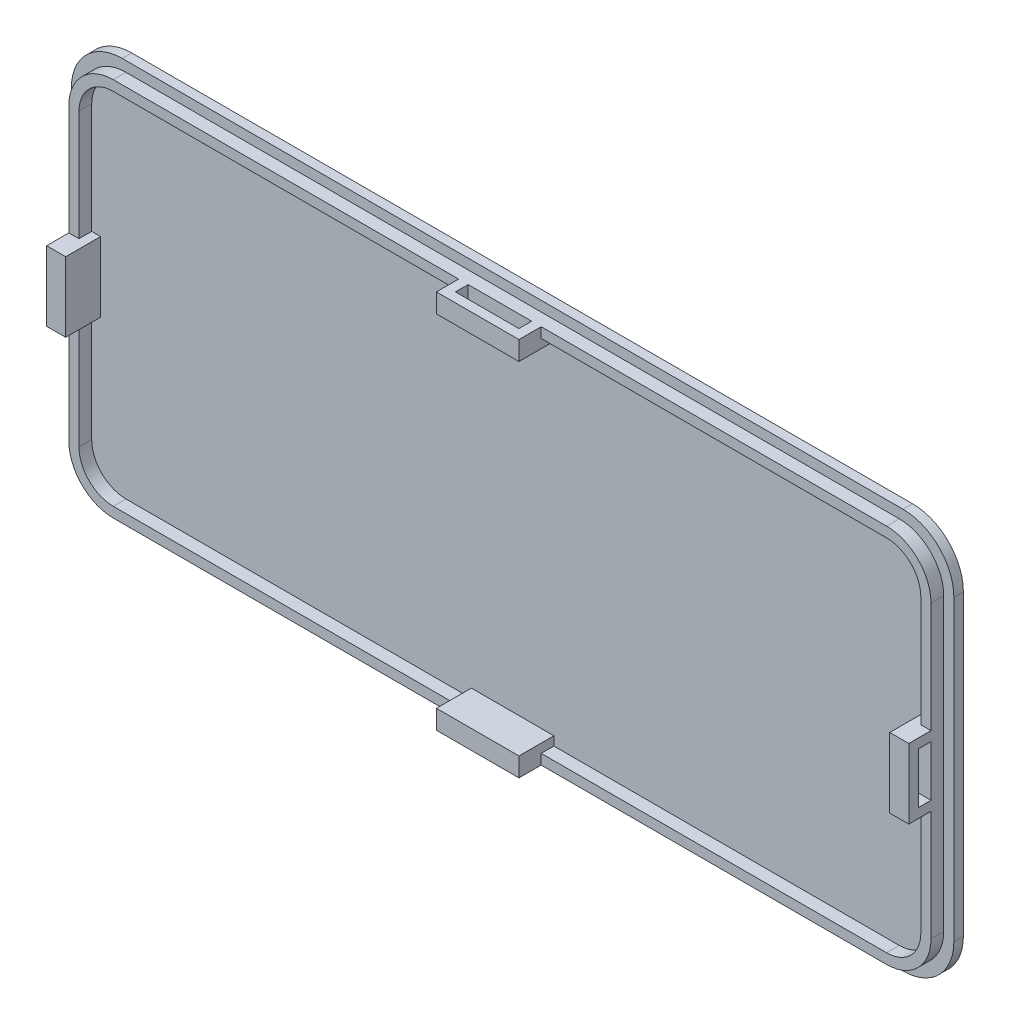
SolidWorks part; units mm, degrees
ref_plane "Front Plane" through (0, 0, 0) normal (0, 0, 1) x (1, 0, 0)
ref_plane "Top Plane" through (0, 0, 0) normal (0, 1, 0) x (1, 0, 0)
ref_plane "Right Plane" through (0, 0, 0) normal (1, 0, 0) x (0, 0, -1)
other "Configuration Table"
sketch "Sketch1" plane through (0, 0, 0) normal (0, 0, 1) x (1, 0, 0)
  line L1 (-61.5, 31.5) -> (61.5, 31.5)
  line L2 (-69.5, 23.5) -> (-69.5, -23.5)
  line L3 (-61.5, -31.5) -> (61.5, -31.5)
  line L4 (69.5, 23.5) -> (69.5, -23.5)
  line L5 (-69.5, 31.5) -> (69.5, -31.5) construction
  line L6 (-69.5, -31.5) -> (69.5, 31.5) construction
  arc A0 (-69.5, -23.5) -> (-61.5, -31.5) centre (-61.5, -23.5) ccw
  arc A1 (61.5, -31.5) -> (69.5, -23.5) centre (61.5, -23.5) ccw
  arc A2 (61.5, 31.5) -> (69.5, 23.5) centre (61.5, 23.5) cw
  arc A3 (-61.5, 31.5) -> (-69.5, 23.5) centre (-61.5, 23.5) ccw
  point P0 (0, 0)
  dimension "D3" = 8
  dimension "D1" = 139
  dimension "D2" = 63
extrude "Boss-Extrude1" add sketch "Sketch1" along normal blind 1.5
sketch "Sketch2" plane through (0, 0, 1.5) normal (0, 0, 1) x (1, 0, 0)
  line L1 (-58, 18) -> (58, 18) construction
  line L2 (-58, 18) -> (-58, -18) construction
  line L3 (-58, -18) -> (58, -18) construction
  line L4 (58, 18) -> (58, -18) construction
  line L5 (-58, 18) -> (58, -18) construction
  line L6 (-58, -18) -> (58, 18) construction
  circle A0 centre (-58, 18) radius 6
  circle A1 centre (-58, 18) radius 5.1
  circle A2 centre (58, 18) radius 6
  circle A3 centre (58, 18) radius 5.1
  circle A4 centre (-58, -18) radius 6
  circle A5 centre (-58, -18) radius 5.1
  circle A6 centre (58, -18) radius 6
  circle A7 centre (58, -18) radius 5.1
  point P0 (0, 0)
  dimension "D1" = 12
  dimension "D2" = 10.2
  dimension "D3" = 116
  dimension "D4" = 36
extrude "Boss-Extrude2" add sketch "Sketch2" against normal blind 1 from offset 1.5 offset against normal yes
sketch "Sketch3" plane through (0, 0, 1.5) normal (0, 0, 1) x (1, 0, 0)
  line L0 (60.9, 29.9) -> (-60.9, 29.9)
  line L1 (-67.9, 22.9) -> (-67.9, -22.9)
  line L2 (-60.9, -29.9) -> (60.9, -29.9)
  line L3 (67.9, -22.9) -> (67.9, 22.9)
  line L16 (61.5, 31.5) -> (-61.5, 31.5) construction
  line L17 (-61.5, -31.5) -> (61.5, -31.5) construction
  line L18 (60.9, 28.3) -> (-60.9, 28.3)
  line L19 (69.5, -23.5) -> (69.5, 23.5) construction
  line L20 (-66.3, 22.9) -> (-66.3, -22.9)
  line L21 (-69.5, 23.5) -> (-69.5, -23.5) construction
  line L22 (-60.9, -28.3) -> (60.9, -28.3)
  line L23 (66.3, -22.9) -> (66.3, 22.9)
  arc A16 (-60.9, 29.9) -> (-67.9, 22.9) centre (-60.9, 22.9) ccw
  arc A17 (60.9, -29.9) -> (67.9, -22.9) centre (60.9, -22.9) ccw
  arc A18 (67.9, 22.9) -> (60.9, 29.9) centre (60.9, 22.9) ccw
  arc A19 (-67.9, -22.9) -> (-60.9, -29.9) centre (-60.9, -22.9) ccw
  arc A20 (-60.9, 28.3) -> (-66.3, 22.9) centre (-60.9, 22.9) ccw
  arc A21 (-66.3, -22.9) -> (-60.9, -28.3) centre (-60.9, -22.9) ccw
  arc A22 (60.9, -28.3) -> (66.3, -22.9) centre (60.9, -22.9) ccw
  arc A23 (66.3, 22.9) -> (60.9, 28.3) centre (60.9, 22.9) ccw
  dimension "D1" = 7
  dimension "D2" = 1.6
  dimension "D3" = 1.6
  dimension "D4" = 1.6
  dimension "D5" = 1.6
  dimension "D6" = 1.6
extrude "Boss-Extrude3" add sketch "Sketch3" along normal blind 2
sketch "Sketch4" plane through (0, 0, 3.5) normal (0, 0, 1) x (1, 0, 0)
  line L0 (60.9, 29.9) -> (-60.9, 29.9) construction
  line L4 (0, -28.15) -> (0, 28.4) construction
  line L7 (-6.5, 26.9) -> (6.5, 26.9)
  line L8 (-6.5, 26.9) -> (-6.5, 29.9)
  line L9 (-6.5, 29.9) -> (6.5, 29.9)
  line L10 (6.5, 26.9) -> (6.5, 29.9)
  line L11 (-6.5, 26.9) -> (6.5, 29.9) construction
  line L12 (-6.5, 29.9) -> (6.5, 26.9) construction
  line L13 (0, 0) -> (0, 22.1365) construction
  line L14 (-66.4, 0) -> (66.4, 0) construction
  line L23 (6.5, -26.9) -> (6.5, -29.9)
  line L24 (-6.5, -29.9) -> (6.5, -29.9)
  line L25 (-6.5, -26.9) -> (6.5, -26.9)
  line L26 (-6.5, -26.9) -> (-6.5, -29.9)
  line L27 (67.9, -22.9) -> (67.9, 22.9) construction
  line L28 (64.9, 5.5) -> (67.9, 5.5)
  line L29 (64.9, 5.5) -> (64.9, -5.5)
  line L30 (64.9, -5.5) -> (67.9, -5.5)
  line L31 (67.9, 5.5) -> (67.9, -5.5)
  line L32 (64.9, 5.5) -> (67.9, -5.5) construction
  line L33 (64.9, -5.5) -> (67.9, 5.5) construction
  line L34 (-64.9, -5.5) -> (-67.9, 5.5) construction
  line L35 (-64.9, 5.5) -> (-67.9, -5.5) construction
  line L36 (-67.9, 5.5) -> (-67.9, -5.5)
  line L37 (-64.9, -5.5) -> (-67.9, -5.5)
  line L38 (-64.9, 5.5) -> (-64.9, -5.5)
  line L39 (-64.9, 5.5) -> (-67.9, 5.5)
  point P0 (0, 0)
  dimension "D1" = 13
  dimension "D2" = 3
  dimension "D3" = 11
  dimension "D4" = 3
extrude "Boss-Extrude4" add sketch "Sketch4" along normal mid plane 7
sketch "Sketch5" plane through (0, 29.9, 0) normal (0, 1, 0) x (1, 0, 0)
  line L0 (0, 0) -> (0, 18.9979) construction
  line L12 (6.5, -7) -> (6.5, -3.5) construction
  line L13 (-5, -3.5) -> (5, -3.5)
  line L14 (-5, -3.5) -> (-5, -5.5)
  line L15 (-5, -5.5) -> (5, -5.5)
  line L16 (5, -3.5) -> (5, -5.5)
  line L17 (-6.5, -7) -> (-6.5, -3.5) construction
  line L18 (-6.5, -3.5) -> (-60.9, -3.5) construction
  dimension "D1" = 1.5
  dimension "D2" = 1.5
  dimension "D3" = 2
extrude "Cut-Extrude1" cut sketch "Sketch5" against normal blind 2
mirror "Mirror1" about plane through (0, 0, 0) normal (0, 1, 0) of "Cut-Extrude1"
sketch "Sketch7" plane through (0, -31.5, 0) normal (0, -1, 0) x (-1, 0, 0)
  line L1 (1, -9.7058) -> (-1, -9.7058)
  line L2 (1, -9.7058) -> (1, 9.7058)
  line L3 (1, 9.7058) -> (-1, 9.7058)
  line L4 (-1, -9.7058) -> (-1, 9.7058)
  line L5 (1, -9.7058) -> (-1, 9.7058) construction
  line L6 (1, 9.7058) -> (-1, -9.7058) construction
  point P0 (0, 0)
  dimension "D1" = 2
extrude "Cut-Extrude3" cut sketch "Sketch7" against normal blind 0.8
sketch "Sketch8" plane through (0, 0, 0) normal (0, 0, -1) x (-1, 0, 0)
  circle A0 centre (-58, 18) radius 5.1
  circle A1 centre (58, 18) radius 5.1
  circle A2 centre (58, -18) radius 5.1
  circle A3 centre (-58, -18) radius 5.1
extrude "Cut-Extrude4" cut sketch "Sketch8" against normal blind 1
sketch "Sketch9" plane through (67.9, 0, 0) normal (1, 0, 0) x (0, 0, -1)
  line L0 (-7, 5.5) -> (-3.5, 5.5) construction
  line L1 (-5.5, 4) -> (-3.5, 4)
  line L2 (-5.5, 4) -> (-5.5, -4)
  line L3 (-5.5, -4) -> (-3.5, -4)
  line L4 (-3.5, 4) -> (-3.5, -4)
  line L5 (-7, -5.5) -> (-3.5, -5.5) construction
  line L6 (-3.5, 5.5) -> (-3.5, 22.9) construction
  dimension "D1" = 1.5
  dimension "D2" = 1.5
  dimension "D3" = 2
extrude "Cut-Extrude5" cut sketch "Sketch9" against normal blind 2
mirror "Mirror2" about plane through (0, 0, 0) normal (1, 0, 0) of "Cut-Extrude5"
